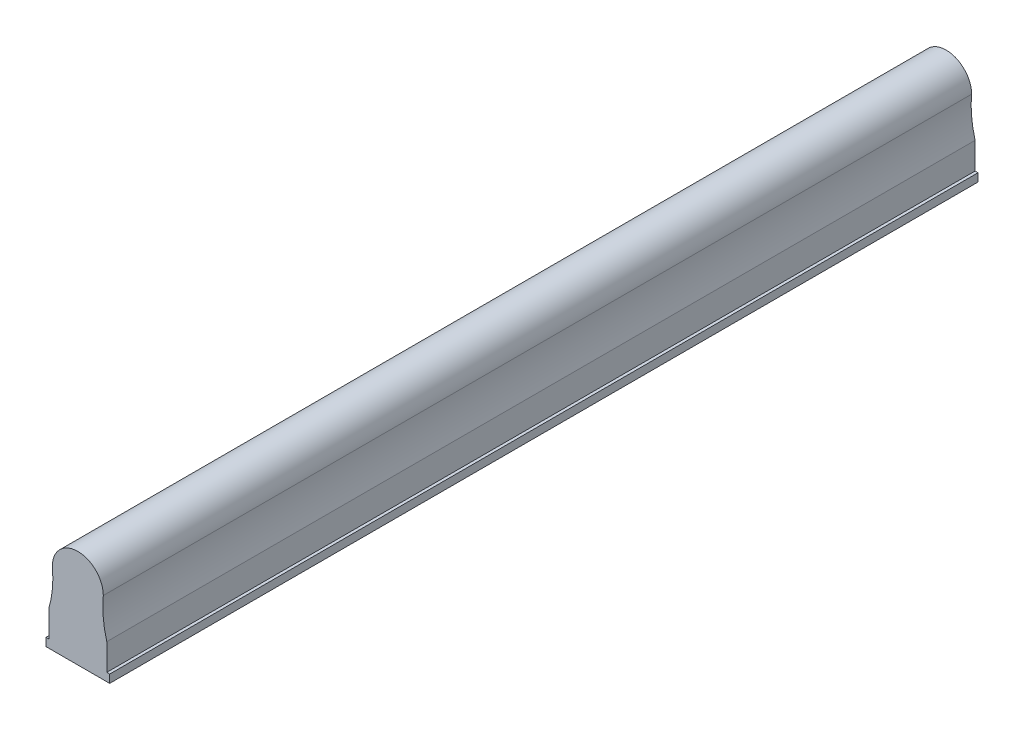
from build123d import *

# Parameters (mm, degrees)
EXTRUDE_1_DEPTH = 300


with BuildPart() as part:
    # 草图1 → 凸台-拉伸1 (new body)
    with BuildSketch(Plane.XY):
        with BuildLine():
            Line((10, 12), (10, 2.8))
            Line((10, 2.8), (11, 2.8))
            Line((11, 2.8), (11, 0))
            Line((11, 0), (-11, 0))
            Line((-11, 0), (-11, 2.8))
            Line((-11, 2.8), (-10, 2.8))
            Line((-10, 2.8), (-10, 12))
            add(Edge.make_bspline(
                [(-8.8, 25.2), (-8.148207528, 18.483731085), (-10, 12)],
                knots=[0, 0, 0, 1, 1, 1], degree=2))
            ThreePointArc((-8.8, 25.2), (0, 34), (8.8, 25.2))
            add(Edge.make_bspline(
                [(8.8, 25.2), (8.148207528, 18.483731085), (10, 12)],
                knots=[0, 0, 0, 1, 1, 1], degree=2))
        make_face()
    extrude(amount=EXTRUDE_1_DEPTH)


solid = part.part
